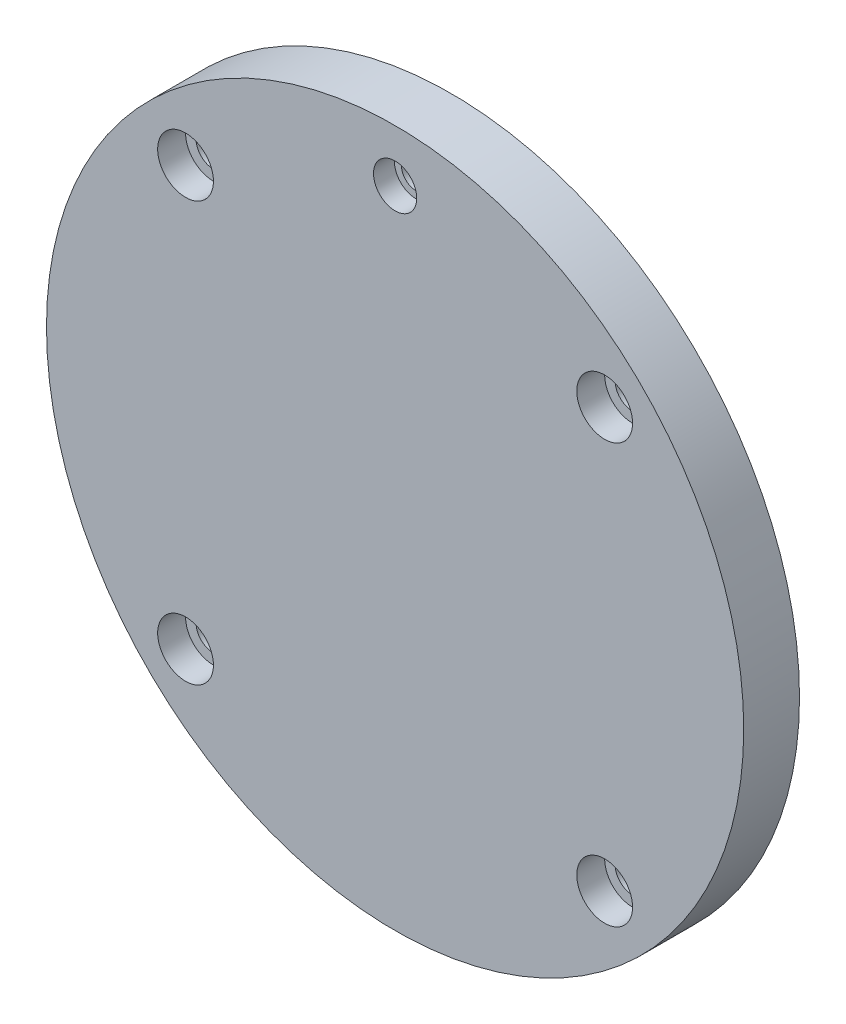
SolidWorks part; units mm, degrees
material "1060-H12 bar (SS)"
ref_plane "Front Plane" through (0, 0, 0) normal (0, 0, 1) x (1, 0, 0)
ref_plane "Top Plane" through (0, 0, 0) normal (0, 1, 0) x (1, 0, 0)
ref_plane "Right Plane" through (0, 0, 0) normal (1, 0, 0) x (0, 0, -1)
sketch "Sketch1" plane through (0, 0, 0) normal (0, 0, 1) x (1, 0, 0)
  circle A0 centre (0, 0) radius 50
extrude "Boss-Extrude1" add sketch "Sketch1" along normal blind 8
sketch "Sketch2" plane through (0, 0, 8) normal (0, 0, 1) x (1, 0, 0)
  line L0 (-50, 0) -> (50, 0) construction
  line L1 (0, 50) -> (0, -50) construction
  line L2 (-53.9261, 30.05) -> (53.7661, 30.05) construction
  line L3 (-54.8863, -30.05) -> (67.6877, -30.05) construction
  circle A0 centre (0, 0) radius 50 construction
  circle A1 centre (0, 0) radius 42.5 construction
  circle A2 centre (-30.0541, 30.05) radius 4
  circle A3 centre (30.0541, 30.05) radius 4
  circle A4 centre (-30.0541, -30.05) radius 4
  circle A5 centre (30.0541, -30.05) radius 4
  dimension "D1" = 30.05
  dimension "D2" = 30.05
extrude "Cut-Extrude1" cut sketch "Sketch2" against normal blind 4
sketch "Sketch3" plane through (0, 0, 8) normal (0, 0, 1) x (1, 0, 0)
  circle A0 centre (0, 0) radius 42.5 construction
  circle A1 centre (0, 42.5) radius 3.1
extrude "Cut-Extrude2" cut sketch "Sketch3" against normal blind 3
sketch "Sketch4" plane through (0, 0, 4) normal (0, 0, 1) x (1, 0, 0)
  circle A0 centre (-30.0541, 30.05) radius 2.5
  circle A1 centre (30.0541, 30.05) radius 2.5
  circle A2 centre (-30.0541, -30.05) radius 2.5
  circle A3 centre (30.0541, -30.05) radius 2.5
  circle A4 centre (0, 42.5) radius 2.1
extrude "Cut-Extrude3" cut sketch "Sketch4" against normal through all
sketch "Sketch5" plane through (0, 0, 5) normal (0, 0, 1) x (1, 0, 0)
  circle A0 centre (0, 42.5) radius 2.1
extrude "Cut-Extrude4" cut sketch "Sketch5" against normal blind 5
